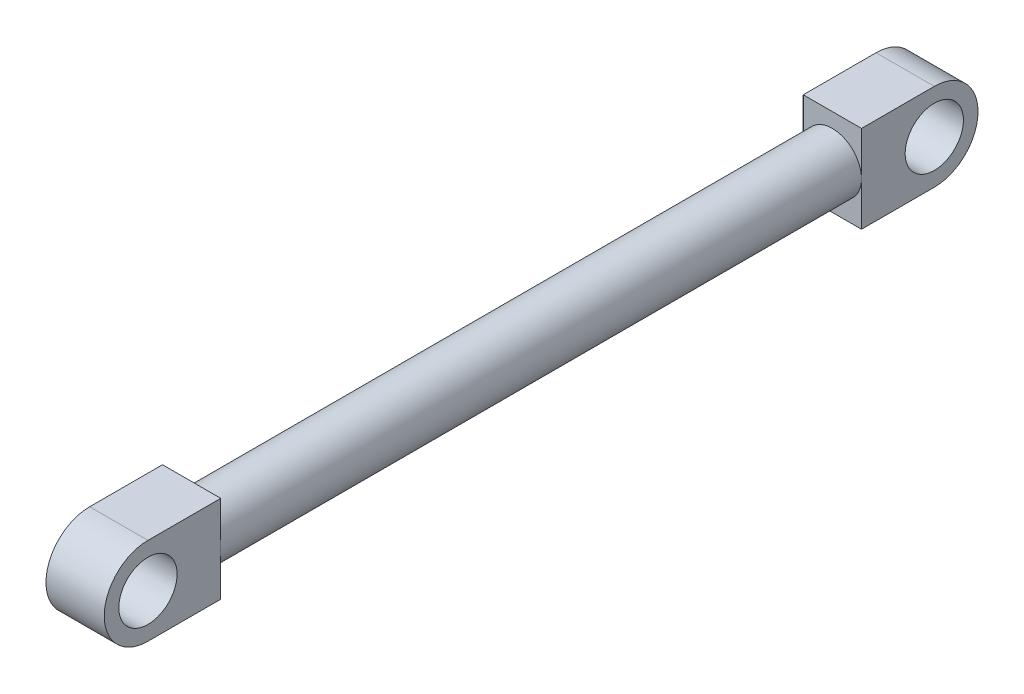
SolidWorks part; units mm, degrees
ref_plane "Front Plane" through (0, 0, 0) normal (0, 0, 1) x (1, 0, 0)
ref_plane "Top Plane" through (0, 0, 0) normal (0, 1, 0) x (1, 0, 0)
ref_plane "Right Plane" through (0, 0, 0) normal (1, 0, 0) x (0, 0, -1)
other "Configuration Table"
sketch "Sketch1" plane through (0, 0, 0) normal (0, 0, 1) x (1, 0, 0)
  circle A0 centre (0, 0) radius 5
  dimension "D1" = 10
extrude "Boss-Extrude1" add sketch "Sketch1" along normal blind 110
sketch "Sketch2" plane through (0, 0, 0) normal (0, 0, -1) x (-1, 0, 0)
  line L1 (-5, 7.5) -> (5, 7.5)
  line L2 (-5, 7.5) -> (-5, -7.5)
  line L3 (-5, -7.5) -> (5, -7.5)
  line L4 (5, 7.5) -> (5, -7.5)
  line L5 (-5, 7.5) -> (5, -7.5) construction
  line L6 (-5, -7.5) -> (5, 7.5) construction
  point P0 (0, 0)
  dimension "D1" = 10
  dimension "D2" = 15
extrude "Boss-Extrude2" add sketch "Sketch2" along normal blind 20
sketch "Sketch3" plane through (0, 0, 110) normal (0, 0, 1) x (1, 0, 0)
  line L1 (-5, -7.5) -> (5, -7.5)
  line L2 (-5, -7.5) -> (-5, 7.5)
  line L3 (-5, 7.5) -> (5, 7.5)
  line L4 (5, -7.5) -> (5, 7.5)
  line L5 (-5, -7.5) -> (5, 7.5) construction
  line L6 (-5, 7.5) -> (5, -7.5) construction
  point P0 (0, 0)
extrude "Boss-Extrude3" add sketch "Sketch3" along normal blind 20
sketch "Sketch4" plane through (5, 0, 0) normal (1, 0, 0) x (0, 0, -1)
  line L0 (-130, -7.5) -> (-130, 7.5) construction
  line L1 (20, 7.5) -> (20, -7.5) construction
  line L2 (12.5, -7.5) -> (27.9572, -19.3446)
  line L3 (27.9572, -19.3446) -> (25.4125, 11.1116)
  line L4 (25.4125, 11.1116) -> (12.5, 7.5)
  line L5 (-122.5, 7.5) -> (-386.4993, 23.053)
  line L6 (-386.4993, 23.053) -> (-390.0049, -19.3446)
  line L7 (-390.0049, -19.3446) -> (-122.5, -7.5)
  circle A0 centre (12.5, 0) radius 5
  arc A1 (12.5, -7.5) -> (12.5, 7.5) centre (12.5, 0) ccw
  circle A2 centre (-122.5, 0) radius 5
  arc A3 (-122.5, 7.5) -> (-122.5, -7.5) centre (-122.5, 0) ccw
  dimension "D1" = 10
  dimension "D2" = 7.5
  dimension "D3" = 10
  dimension "D4" = 7.5
extrude "Cut-Extrude1" cut sketch "Sketch4" against normal through all
